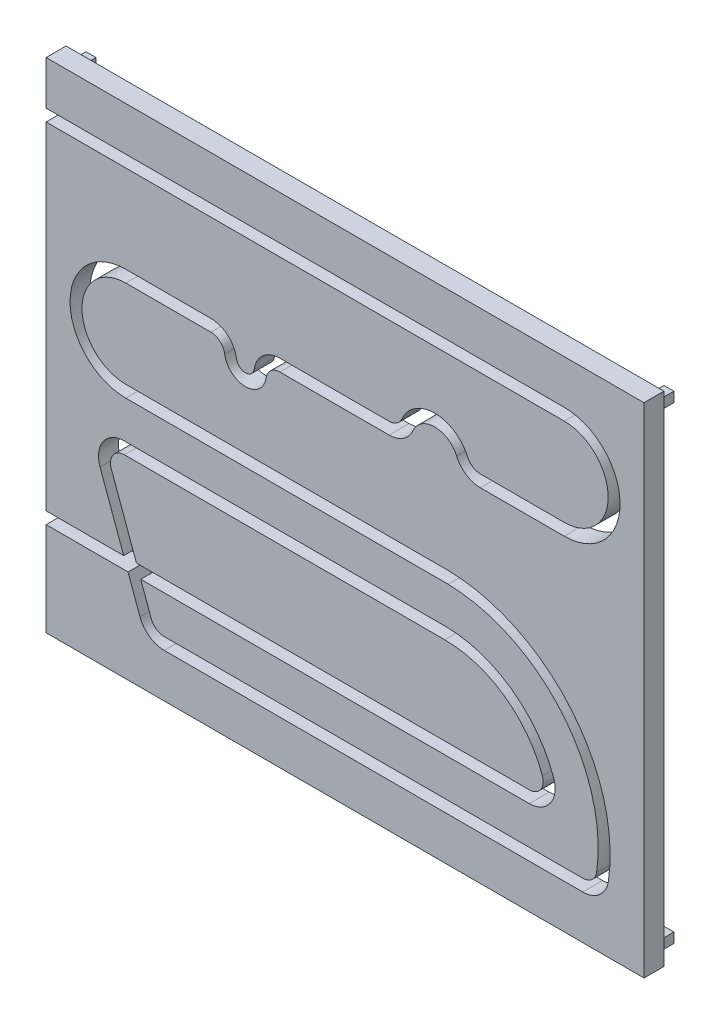
SolidWorks part; units mm, degrees
ref_plane "Front Plane" through (0, 0, 0) normal (0, 0, 1) x (1, 0, 0)
ref_plane "Top Plane" through (0, 0, 0) normal (0, 1, 0) x (1, 0, 0)
ref_plane "Right Plane" through (0, 0, 0) normal (1, 0, 0) x (0, 0, -1)
sketch "Sketch1" plane through (0, 0, 0) normal (0, 0, 1) x (1, 0, 0)
  line L1 (-300, 250) -> (300, 250)
  line L2 (-300, 250) -> (-300, -250)
  line L3 (-300, -250) -> (300, -250)
  line L4 (300, 250) -> (300, -250)
  line L5 (-300, 250) -> (300, -250) construction
  line L6 (-300, -250) -> (300, 250) construction
  point P0 (0, 0)
  dimension "D1" = 500
  dimension "D2" = 600
extrude "Boss-Extrude1" add sketch "Sketch1" along normal blind 20
sketch "Sketch2" plane through (0, 0, 20) normal (0, 0, 1) x (1, 0, 0)
  line L0 (-300, 0) -> (300, 0) construction
  line L1 (-300, 250) -> (-300, -250) construction
  line L2 (300, -250) -> (300, 250) construction
  line L3 (0, 250) -> (0, -250) construction
  line L4 (300, 250) -> (-300, 250) construction
  line L5 (-300, -250) -> (300, -250) construction
  line L6 (-300, 199.9611) -> (220, 199.9611)
  line L7 (220, 99.9611) -> (135.8258, 99.9611)
  line L8 (-220, -0.0389) -> (103.529, -0.0389)
  line L9 (44.1742, 99.9611) -> (-2.0406, 99.9611)
  line L10 (-134.641, 99.9611) -> (-220, 99.9611)
  line L11 (-100, 99.9611) -> (-100, 100) construction
  line L12 (-65.359, 99.9611) -> (-2.0406, 99.9611)
  line L13 (238.5641, -200) -> (-181.4003, -200)
  line L14 (-200.1942, -186.8404) -> (-240.2309, -76.8404)
  line L15 (-221.437, -50) -> (100, -50)
  line L16 (184.8528, -150) -> (-300, -150) construction
  arc A0 (220, 199.9611) -> (220, 99.9611) centre (220, 149.9611) cw
  arc A1 (-220, 99.9611) -> (-220, -0.0389) centre (-220, 49.9611) ccw
  arc A2 (117.4955, 111.9611) -> (62.5045, 111.9611) centre (90, 99.9611) ccw
  arc A4 (-114.8461, 82.8182) -> (-85.1539, 82.8182) centre (-100, 84.9611) ccw
  arc A5 (135.8258, 99.9611) -> (117.4955, 111.9611) centre (135.8258, 119.9611) cw
  arc A7 (44.1742, 99.9611) -> (62.5045, 111.9611) centre (44.1742, 119.9611) ccw
  arc A9 (-114.8461, 82.8182) -> (-134.641, 99.9611) centre (-134.641, 79.9611) ccw
  arc A11 (103.529, -0.0389) -> (258.3589, -182.8571) centre (100, -160) cw
  arc A12 (-85.1539, 82.8182) -> (-65.359, 99.9611) centre (-65.359, 79.9611) cw
  arc A13 (100, -50) -> (203.709, -123.3333) centre (100, -160) cw
  arc A14 (-181.4003, -200) -> (-200.1942, -186.8404) centre (-181.4003, -180) cw
  arc A15 (-240.2309, -76.8404) -> (-221.437, -50) centre (-221.437, -70) cw
  arc A16 (203.709, -123.3333) -> (184.8528, -150) centre (184.8528, -130) cw
  arc A17 (238.5641, -200) -> (258.3589, -182.8571) centre (238.5641, -180) ccw
  point P51 (-250, -50)
  dimension "D1" = 50
  dimension "D2" = 50
  dimension "D3" = 160
  dimension "D4" = 60
  dimension "D5" = 30
  dimension "D6" = 220
  dimension "D7" = 20
  dimension "D8" = 20
  dimension "D9" = 440
  dimension "D10" = 90
  dimension "D12" = 100
  dimension "D14" = 50
  dimension "D17" = 110
  dimension "D20" = 90
  dimension "D21" = 100
  dimension "D22" = 20
  dimension "D11" = 100
  dimension "D13" = 90
  dimension "D15" = 50
  dimension "D16" = 110
  dimension "D18" = 50
  dimension "D19" = 50
extrude "Cut-Extrude-Thin1" cut sketch "Sketch2" against normal blind 20 and the other way through all thin thin type mid plane wall 12
sketch "Sketch3" plane through (0, 0, 20) normal (0, 0, 1) x (1, 0, 0)
  line L0 (-300, -150) -> (184.8528, -150)
  line L1 (184.8528, -150) -> (-300, -150) construction
extrude "Cut-Extrude-Thin2" cut sketch "Sketch3" against normal blind 20 and the other way through all thin thin type mid plane wall 12
sketch "Sketch4" plane through (0, 0, 0) normal (0, 0, -1) x (-1, 0, 0)
  line L0 (-300, -250) -> (-300, 250) construction
  line L1 (-295, 240) -> (-285, 240)
  line L2 (-295, 240) -> (-295, 230)
  line L3 (-295, 230) -> (-285, 230)
  line L4 (-285, 240) -> (-285, 230)
  line L5 (-295, 240) -> (-285, 230) construction
  line L6 (-295, 230) -> (-285, 240) construction
  line L7 (-300, 250) -> (300, 250) construction
  point P0 (-290, 235)
  dimension "D1" = 10
  dimension "D2" = 5
  dimension "D3" = 10
extrude "Boss-Extrude2" add sketch "Sketch4" along normal blind 15
mirror "Mirror1" about plane through (0, 0, 0) normal (1, 0, 0) of "Boss-Extrude2"
mirror "Mirror2" about plane through (0, 0, 0) normal (0, 1, 0) of "Mirror1", "Boss-Extrude2"
sketch "Sketch6" [suppressed] plane through (0, 0, 20) normal (0, 0, 1) x (1, 0, 0)
  line L0 (220, 205.9611) -> (-300, 205.9611) construction
  line L1 (220, 205.9611) -> (-300, 205.9611)
  line L2 (220, 93.9611) -> (135.8258, 93.9611) construction
  line L3 (44.1742, 93.9611) -> (-65.359, 93.9611) construction
  line L4 (-134.641, 93.9611) -> (-220, 93.9611) construction
  line L5 (-220, 5.9611) -> (103.5946, 5.9611) construction
  line L6 (220, 93.9611) -> (135.8258, 93.9611)
  line L7 (44.1742, 93.9611) -> (-65.359, 93.9611)
  line L8 (-134.641, 93.9611) -> (-220, 93.9611)
  line L9 (-220, 5.9611) -> (103.5946, 5.9611)
  line L10 (-217.8042, -156) -> (-300, -156) construction
  line L11 (-205.8323, -188.8925) -> (-217.8042, -156) construction
  line L12 (238.5641, -206) -> (-181.4003, -206) construction
  line L13 (-217.8042, -156) -> (-300, -156)
  line L14 (-205.8323, -188.8925) -> (-217.8042, -156)
  line L15 (238.5641, -206) -> (-181.4003, -206)
  line L16 (-228.3073, -171) -> (-300, -171)
  line L17 (-219.9277, -194.0228) -> (-228.3073, -171)
  line L18 (238.5641, -221) -> (-181.4003, -221)
  line L19 (-220, 20.9611) -> (103.7535, 20.9611)
  line L20 (-135.4965, 78.9611) -> (-220, 78.9611)
  line L21 (44.1742, 78.9611) -> (-64.5035, 78.9611)
  line L22 (220, 78.9611) -> (135.8258, 78.9611)
  line L23 (220, 220.9611) -> (-300, 220.9611)
  line L24 (-300, -171) -> (-300, -156)
  line L25 (-300, 205.9611) -> (-300, 220.9611)
  arc A0 (220, 93.9611) -> (220, 205.9611) centre (220, 149.9611) ccw construction
  arc A1 (111.9964, 109.5611) -> (135.8258, 93.9611) centre (135.8258, 119.9611) ccw construction
  arc A2 (-65.359, 93.9611) -> (-79.2154, 81.9611) centre (-65.359, 79.9611) ccw construction
  arc A3 (-120.7846, 81.9611) -> (-134.641, 93.9611) centre (-134.641, 79.9611) ccw construction
  arc A4 (44.1742, 93.9611) -> (68.0036, 109.5611) centre (44.1742, 119.9611) ccw construction
  arc A5 (111.9964, 109.5611) -> (68.0036, 109.5611) centre (90, 99.9611) ccw construction
  arc A6 (-120.7846, 81.9611) -> (-79.2154, 81.9611) centre (-100, 84.9611) ccw construction
  arc A7 (-220, 93.9611) -> (-220, 5.9611) centre (-220, 49.9611) ccw construction
  arc A8 (220, 93.9611) -> (220, 205.9611) centre (220, 149.9611) ccw
  arc A9 (111.9964, 109.5611) -> (135.8258, 93.9611) centre (135.8258, 119.9611) ccw
  arc A10 (-65.359, 93.9611) -> (-79.2154, 81.9611) centre (-65.359, 79.9611) ccw
  arc A11 (-120.7846, 81.9611) -> (-134.641, 93.9611) centre (-134.641, 79.9611) ccw
  arc A12 (44.1742, 93.9611) -> (68.0036, 109.5611) centre (44.1742, 119.9611) ccw
  arc A13 (111.9964, 109.5611) -> (68.0036, 109.5611) centre (90, 99.9611) ccw
  arc A14 (-120.7846, 81.9611) -> (-79.2154, 81.9611) centre (-100, 84.9611) ccw
  arc A15 (-220, 93.9611) -> (-220, 5.9611) centre (-220, 49.9611) ccw
  arc A16 (-205.8323, -188.8925) -> (-181.4003, -206) centre (-181.4003, -180) ccw construction
  arc A17 (238.5641, -206) -> (264.2974, -183.7143) centre (238.5641, -180) ccw construction
  arc A18 (264.2974, -183.7143) -> (103.5946, 5.9611) centre (100, -160) ccw construction
  arc A19 (-205.8323, -188.8925) -> (-181.4003, -206) centre (-181.4003, -180) ccw
  arc A20 (238.5641, -206) -> (264.2974, -183.7143) centre (238.5641, -180) ccw
  arc A21 (264.2974, -183.7143) -> (103.5946, 5.9611) centre (100, -160) ccw
  arc A22 (-219.9277, -194.0228) -> (-181.4003, -221) centre (-181.4003, -180) ccw
  arc A23 (238.5641, -221) -> (279.1435, -185.8571) centre (238.5641, -180) ccw
  arc A24 (279.1435, -185.8571) -> (103.7535, 20.9611) centre (100, -160) ccw
  arc A25 (-220, 78.9611) -> (-220, 20.9611) centre (-220, 49.9611) ccw
  arc A26 (-135.4965, 78.9611) -> (-135.4965, 78.9611) centre (-135.4965, 78.9611) ccw
  arc A27 (-135.4965, 78.9611) -> (-64.5035, 78.9611) centre (-100, 84.9611) ccw
  arc A28 (-64.5035, 78.9611) -> (-64.5035, 78.9611) centre (-64.5035, 78.9611) ccw
  arc A29 (44.1742, 78.9611) -> (81.7514, 103.5611) centre (44.1742, 119.9611) ccw
  arc A30 (98.2486, 103.5611) -> (81.7514, 103.5611) centre (90, 99.9611) ccw
  arc A31 (98.2486, 103.5611) -> (135.8258, 78.9611) centre (135.8258, 119.9611) ccw
  arc A32 (220, 78.9611) -> (220, 220.9611) centre (220, 149.9611) ccw
  dimension "D1" = 15
extrude "Boss-Extrude5" [suppressed] add sketch "Sketch6" along normal blind 0.2
sketch "Sketch7" [suppressed] plane through (0, 0, 20) normal (0, 0, 1) x (1, 0, 0)
  line L0 (220, 193.9611) -> (-300, 193.9611) construction
  line L1 (220, 193.9611) -> (-300, 193.9611)
  line L2 (184.8528, -156) -> (-205.0341, -156) construction
  line L3 (-194.556, -184.7883) -> (-205.0341, -156) construction
  line L4 (238.5641, -194) -> (-181.4003, -194) construction
  line L5 (-220, -6.0389) -> (103.4622, -6.0389) construction
  line L6 (220, 105.9611) -> (135.8258, 105.9611) construction
  line L7 (44.1742, 105.9611) -> (-65.359, 105.9611) construction
  line L8 (184.8528, -156) -> (-205.0341, -156)
  line L9 (-194.556, -184.7883) -> (-205.0341, -156)
  line L10 (238.5641, -194) -> (-181.4003, -194)
  line L11 (-220, -6.0389) -> (103.4622, -6.0389)
  line L12 (220, 105.9611) -> (135.8258, 105.9611)
  line L13 (44.1742, 105.9611) -> (-65.359, 105.9611)
  line L14 (-222.1719, -144) -> (-300, -144) construction
  line L15 (-222.1719, -144) -> (-245.869, -78.8925) construction
  line L16 (-209.4017, -144) -> (-234.5927, -74.7883) construction
  line L17 (184.8528, -144) -> (-209.4017, -144) construction
  line L18 (-221.437, -56) -> (100, -56) construction
  line L19 (-221.437, -44) -> (100, -44) construction
  line L20 (-222.1719, -144) -> (-300, -144)
  line L21 (-222.1719, -144) -> (-245.869, -78.8925)
  line L22 (-209.4017, -144) -> (-234.5927, -74.7883)
  line L23 (184.8528, -144) -> (-209.4017, -144)
  line L24 (-221.437, -56) -> (100, -56)
  line L25 (-221.437, -44) -> (100, -44)
  line L26 (-134.641, 105.9611) -> (-220, 105.9611) construction
  line L27 (-134.641, 105.9611) -> (-220, 105.9611)
  line L28 (220, 178.9611) -> (-300, 178.9611)
  line L29 (220, 120.9611) -> (136.4758, 120.9611)
  line L30 (43.5242, 120.9611) -> (-65.359, 120.9611)
  line L31 (-134.641, 120.9611) -> (-220, 120.9611)
  line L32 (-220, -21.0389) -> (103.2893, -21.0389)
  line L33 (237.6953, -179) -> (-180.7001, -179)
  line L34 (-180.7001, -179) -> (-183.6119, -171)
  line L35 (184.8528, -171) -> (-183.6119, -171)
  line L36 (-221.437, -29) -> (100, -29)
  line L37 (-243.5941, -129) -> (-259.9644, -84.0228)
  line L38 (-243.5941, -129) -> (-300, -129)
  line L39 (-300, -129) -> (-300, -144)
  line L40 (-300, 178.9611) -> (-300, 193.9611)
  arc A0 (220, 105.9611) -> (220, 193.9611) centre (220, 149.9611) ccw construction
  arc A1 (220, 105.9611) -> (220, 193.9611) centre (220, 149.9611) ccw
  arc A2 (-194.556, -184.7883) -> (-181.4003, -194) centre (-181.4003, -180) ccw construction
  arc A3 (238.5641, -194) -> (252.4205, -182) centre (238.5641, -180) ccw construction
  arc A4 (252.4205, -182) -> (103.4622, -6.0389) centre (100, -160) ccw construction
  arc A5 (-220, 105.9611) -> (-220, -6.0389) centre (-220, 49.9611) ccw construction
  arc A6 (122.9945, 114.3611) -> (135.8258, 105.9611) centre (135.8258, 119.9611) ccw construction
  arc A7 (44.1742, 105.9611) -> (57.0055, 114.3611) centre (44.1742, 119.9611) ccw construction
  arc A8 (122.9945, 114.3611) -> (57.0055, 114.3611) centre (90, 99.9611) ccw construction
  arc A9 (-65.359, 105.9611) -> (-91.0923, 83.6754) centre (-65.359, 79.9611) ccw construction
  arc A10 (-108.9077, 83.6754) -> (-91.0923, 83.6754) centre (-100, 84.9611) ccw construction
  arc A11 (-194.556, -184.7883) -> (-181.4003, -194) centre (-181.4003, -180) ccw
  arc A12 (238.5641, -194) -> (252.4205, -182) centre (238.5641, -180) ccw
  arc A13 (252.4205, -182) -> (103.4622, -6.0389) centre (100, -160) ccw
  arc A14 (-220, 105.9611) -> (-220, -6.0389) centre (-220, 49.9611) ccw
  arc A15 (122.9945, 114.3611) -> (135.8258, 105.9611) centre (135.8258, 119.9611) ccw
  arc A16 (44.1742, 105.9611) -> (57.0055, 114.3611) centre (44.1742, 119.9611) ccw
  arc A17 (122.9945, 114.3611) -> (57.0055, 114.3611) centre (90, 99.9611) ccw
  arc A18 (-65.359, 105.9611) -> (-91.0923, 83.6754) centre (-65.359, 79.9611) ccw
  arc A19 (-108.9077, 83.6754) -> (-91.0923, 83.6754) centre (-100, 84.9611) ccw
  arc A20 (-221.437, -44) -> (-245.869, -78.8925) centre (-221.437, -70) ccw construction
  arc A21 (-221.437, -56) -> (-234.5927, -74.7883) centre (-221.437, -70) ccw construction
  arc A22 (184.8528, -144) -> (198.0521, -125.3333) centre (184.8528, -130) ccw construction
  arc A23 (198.0521, -125.3333) -> (100, -56) centre (100, -160) ccw construction
  arc A24 (209.3658, -121.3333) -> (100, -44) centre (100, -160) ccw construction
  arc A25 (184.8528, -156) -> (209.3658, -121.3333) centre (184.8528, -130) ccw construction
  arc A26 (-221.437, -44) -> (-245.869, -78.8925) centre (-221.437, -70) ccw
  arc A27 (-221.437, -56) -> (-234.5927, -74.7883) centre (-221.437, -70) ccw
  arc A28 (184.8528, -144) -> (198.0521, -125.3333) centre (184.8528, -130) ccw
  arc A29 (198.0521, -125.3333) -> (100, -56) centre (100, -160) ccw
  arc A30 (209.3658, -121.3333) -> (100, -44) centre (100, -160) ccw
  arc A31 (184.8528, -156) -> (209.3658, -121.3333) centre (184.8528, -130) ccw
  arc A32 (-108.9077, 83.6754) -> (-134.641, 105.9611) centre (-134.641, 79.9611) ccw construction
  arc A33 (-108.9077, 83.6754) -> (-134.641, 105.9611) centre (-134.641, 79.9611) ccw
  arc A34 (220, 120.9611) -> (220, 178.9611) centre (220, 149.9611) ccw
  arc A35 (136.4758, 120.9611) -> (136.4758, 120.9611) centre (136.4758, 120.9611) ccw
  arc A36 (136.4758, 120.9611) -> (43.5242, 120.9611) centre (90, 99.9611) ccw
  arc A37 (43.5242, 120.9611) -> (43.5242, 120.9611) centre (43.5242, 120.9611) ccw
  arc A38 (-65.359, 120.9611) -> (-100, 101.8928) centre (-65.359, 79.9611) ccw
  arc A39 (-100, 101.8928) -> (-100, 101.8928) centre (-100, 101.8928) ccw
  arc A40 (-100, 101.8928) -> (-134.641, 120.9611) centre (-134.641, 79.9611) ccw
  arc A41 (-220, 120.9611) -> (-220, -21.0389) centre (-220, 49.9611) ccw
  arc A42 (237.6953, -179) -> (103.2893, -21.0389) centre (100, -160) ccw
  arc A43 (237.6953, -179) -> (237.6953, -179) centre (237.6953, -179) ccw
  arc A44 (-180.7001, -179) -> (-180.7001, -179) centre (-180.7001, -179) ccw
  arc A45 (184.8528, -171) -> (223.508, -116.3333) centre (184.8528, -130) ccw
  arc A46 (223.508, -116.3333) -> (100, -29) centre (100, -160) ccw
  arc A47 (-221.437, -29) -> (-259.9644, -84.0228) centre (-221.437, -70) ccw
  dimension "D1" = 15
extrude "Boss-Extrude6" [suppressed] add sketch "Sketch7" along normal blind 0.2
sketch "Sketch9" [suppressed] plane through (0, 0, 20.2) normal (0, 0, 1) x (1, 0, 0)
  line L0 (-234.5927, -74.7883) -> (-209.4017, -144) construction
  line L1 (-209.4017, -144) -> (184.8528, -144) construction
  line L2 (100, -56) -> (-221.437, -56) construction
  line L3 (-234.5927, -74.7883) -> (-209.4017, -144)
  line L4 (-209.4017, -144) -> (184.8528, -144)
  line L5 (100, -56) -> (-221.437, -56)
  line L6 (100, -60.5) -> (-221.437, -60.5)
  line L7 (-230.3641, -73.2492) -> (-206.2508, -139.5)
  line L8 (-206.2508, -139.5) -> (184.8528, -139.5)
  arc A0 (198.0521, -125.3333) -> (100, -56) centre (100, -160) ccw construction
  arc A1 (184.8528, -144) -> (198.0521, -125.3333) centre (184.8528, -130) ccw construction
  arc A2 (-221.437, -56) -> (-234.5927, -74.7883) centre (-221.437, -70) ccw construction
  arc A3 (198.0521, -125.3333) -> (100, -56) centre (100, -160) ccw
  arc A4 (184.8528, -144) -> (198.0521, -125.3333) centre (184.8528, -130) ccw
  arc A5 (-221.437, -56) -> (-234.5927, -74.7883) centre (-221.437, -70) ccw
  arc A6 (-221.437, -60.5) -> (-230.3641, -73.2492) centre (-221.437, -70) ccw
  arc A7 (184.8528, -139.5) -> (193.8095, -126.8333) centre (184.8528, -130) ccw
  arc A8 (193.8095, -126.8333) -> (100, -60.5) centre (100, -160) ccw
  dimension "D1" = 4.5
extrude "Boss-Extrude7" [suppressed] add sketch "Sketch9" along normal blind 0.2
